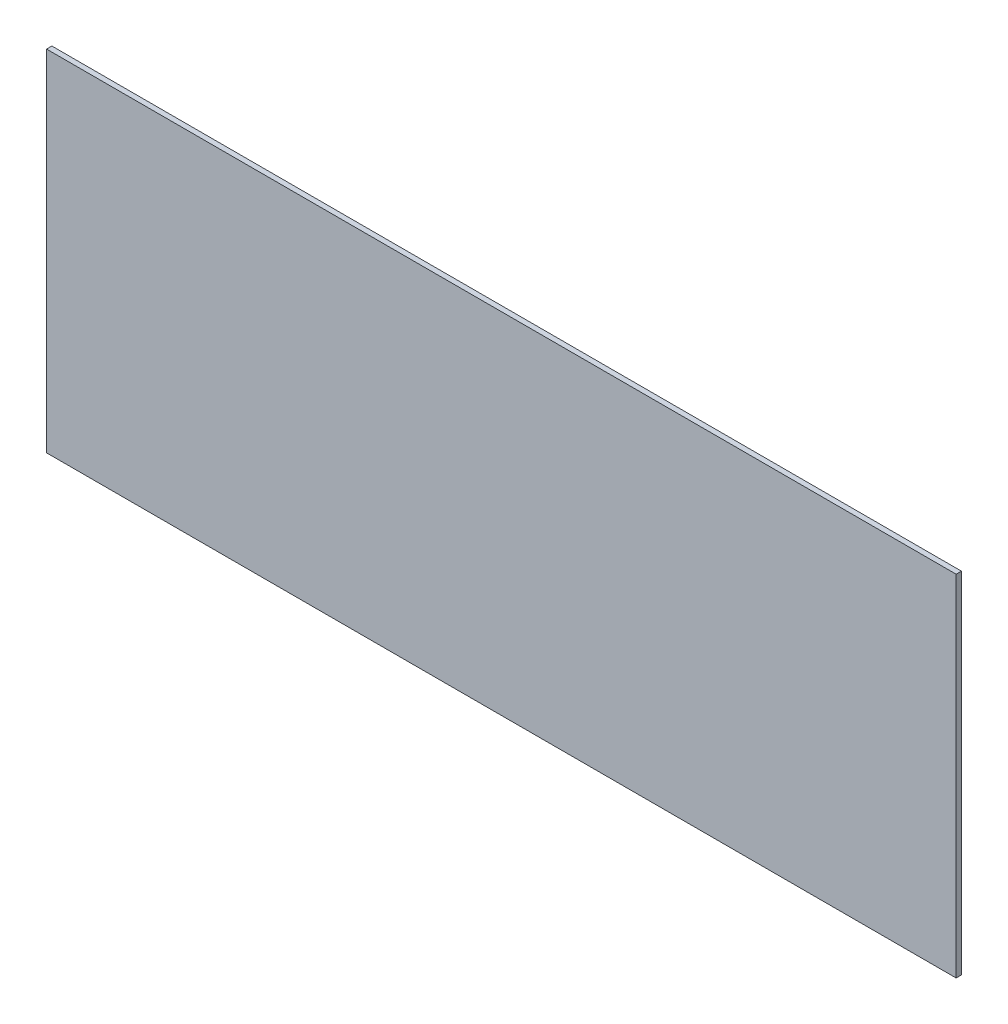
from build123d import *

# Parameters (mm, degrees)
SKETCH1_W           = 515
SKETCH1_H           = 198
BOSS_EXTRUDE1_DEPTH = 3


with BuildPart() as part:
    # Sketch1 → Boss-Extrude1 (new body)
    with BuildSketch(Plane.XY):
        Rectangle(SKETCH1_W, SKETCH1_H)
    extrude(amount=BOSS_EXTRUDE1_DEPTH)


solid = part.part
